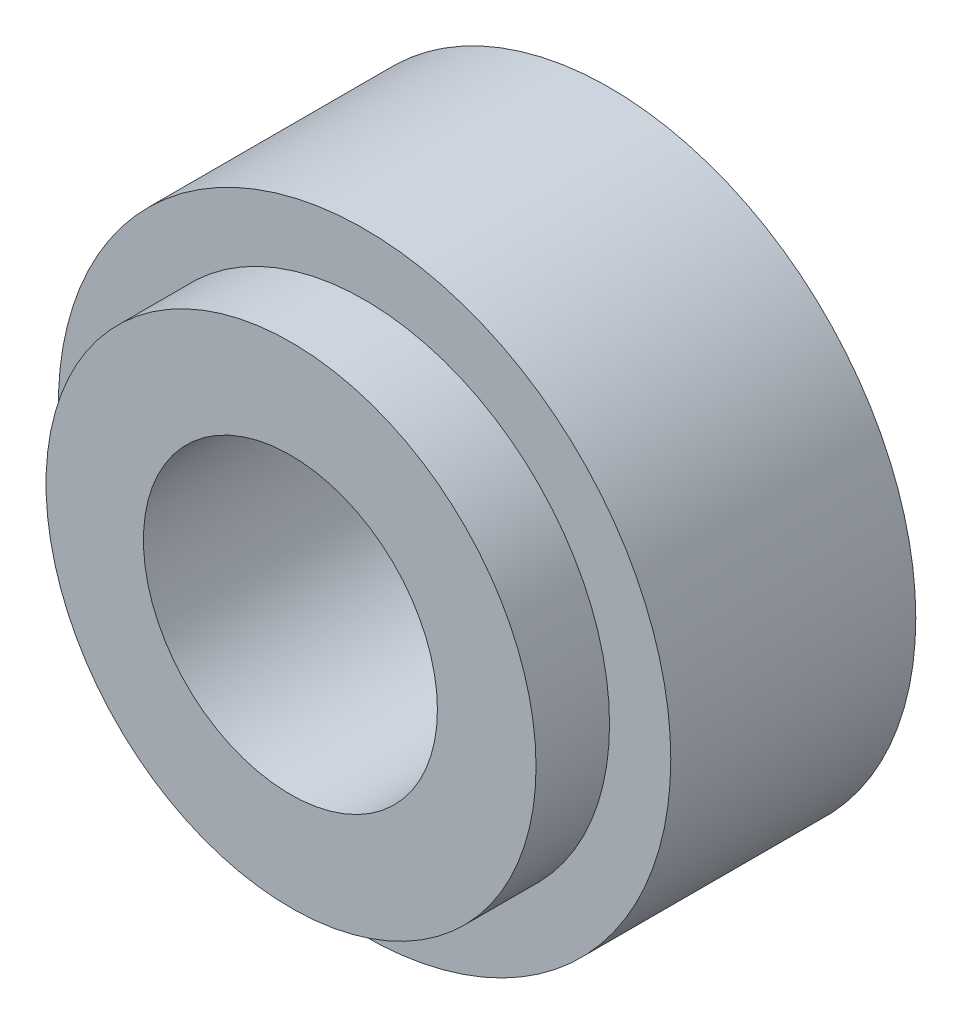
SolidWorks part; units mm, degrees
ref_plane "Front Plane" through (0, 0, 0) normal (0, 0, 1) x (1, 0, 0)
ref_plane "Top Plane" through (0, 0, 0) normal (0, 1, 0) x (1, 0, 0)
ref_plane "Right Plane" through (0, 0, 0) normal (1, 0, 0) x (0, 0, -1)
sketch "Sketch1" plane through (0, 0, 0) normal (0, 0, 1) x (1, 0, 0)
  circle A0 centre (0, 0) radius 12.5
extrude "Boss-Extrude1" add sketch "Sketch1" along normal blind 10
sketch "Sketch2" plane through (0, 0, 10) normal (0, 0, 1) x (1, 0, 0)
  circle A0 centre (0, 0) radius 10
extrude "Boss-Extrude2" add sketch "Sketch2" along normal blind 3
sketch "Sketch12" plane through (0, 0, 13) normal (0, 0, 1) x (1, 0, 0)
  circle A0 centre (0, 0) radius 6.15
hole_wizard "M14 Tapped Hole1" positions "3DSketch8" profile "Sketch13" tap size "M14" standard "Gb"
sketch3d "3DSketch8"
  point P0 (0, 0, 0)
  point P3 (0, 0, 0)
  point P5 (0, 0, 0)
  point P7 (-0.0249, -0.003, 13)
sketch "Sketch13" plane through (-0.0249, -0.003, 13) normal (1, 0, 0) x (0, -1, 0)
  line L0 (0, 0) -> (0, 37.6052)
  line L1 (0, 37.6052) -> (6, 34)
  line L2 (6, 34) -> (6, 0)
  line L5 (6, 0) -> (0, 0)
  line L10 (0, 37.6052) -> (-6, 34) construction
  line L11 (0, -6.35) -> (0, 107.95) construction
  dimension "螺纹孔钻头直径" = 12
  dimension "螺纹孔钻头深度" = 34
  dimension "导头角度" = 118
cosmetic thread "Hole Thread1" parameters "D1"=13, "D2"=14
cosmetic thread "Hole Thread2" parameters "D1"=13, "D2"=14
cosmetic thread "Hole Thread3" parameters "D1"=13, "D2"=14
cosmetic thread "Hole Thread4" parameters "D1"=13, "D2"=14
